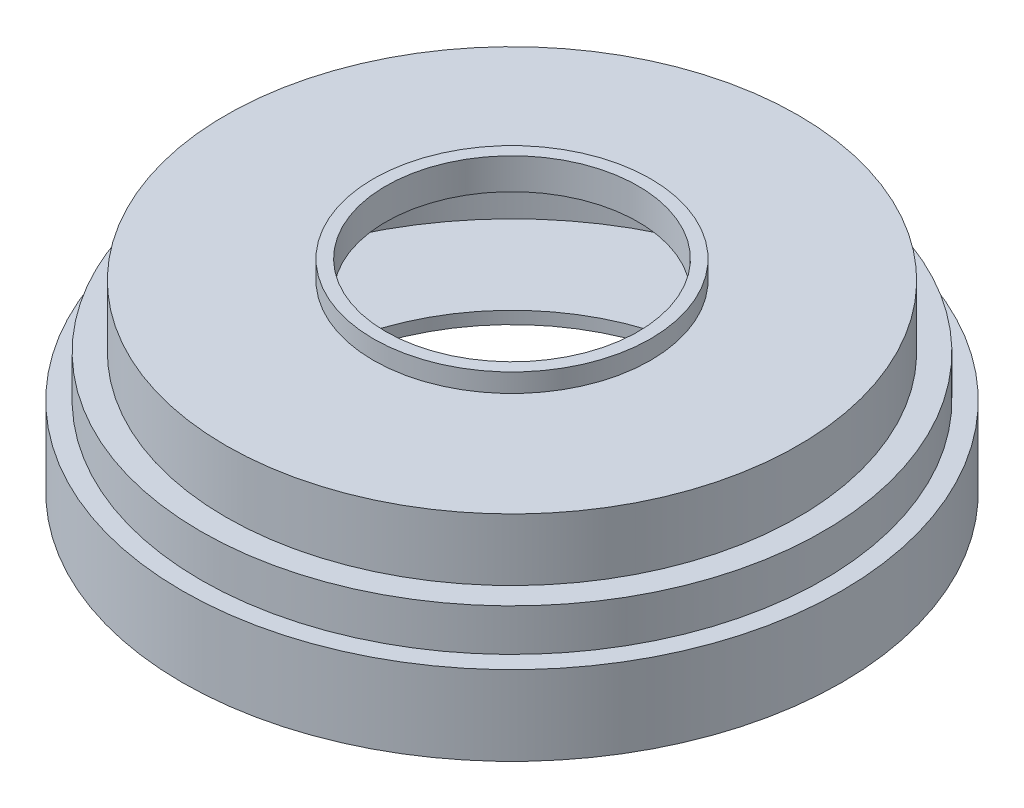
SolidWorks part; units mm, degrees
ref_plane "Front Plane" through (0, 0, 0) normal (0, 0, 1) x (1, 0, 0)
ref_plane "Top Plane" through (0, 0, 0) normal (0, 1, 0) x (1, 0, 0)
ref_plane "Right Plane" through (0, 0, 0) normal (1, 0, 0) x (0, 0, -1)
sketch "Sketch1" plane through (0, 0, 0) normal (0, 0, 1) x (1, 0, 0)
  line L0 (0, 0) -> (0, -21.981) construction
  line L1 (43, 136) -> (43, 141)
  line L2 (-43, 136) -> (43, 136) construction
  line L3 (-55, 136) -> (55, 136) construction
  line L4 (43, 141) -> (-43, 141) construction
  line L5 (60, 141) -> (-60, 141) construction
  line L6 (43, 141) -> (53, 141)
  line L7 (53, 141) -> (53, 153.7728)
  line L9 (53, 153.7728) -> (50, 153.7728)
  line L10 (50, 153.7728) -> (50, 160.5319)
  line L11 (63.1935, 160.5319) -> (-63.1935, 160.5319) construction
  line L12 (50, 160.5319) -> (46, 160.5319)
  line L13 (46, 160.5319) -> (46, 170.5)
  line L14 (106, 170.5) -> (-106, 170.5) construction
  line L15 (46, 170.5) -> (22.2841, 170.5)
  line L16 (22.2841, 170.5) -> (22.2841, 173.5)
  line L17 (41, 136) -> (41, 141)
  line L18 (41, 143) -> (51, 143)
  line L19 (51, 143) -> (51, 151.7728)
  line L20 (51, 151.7728) -> (48, 151.7728)
  line L21 (48, 151.7728) -> (48, 158.5319)
  line L22 (48, 158.5319) -> (44, 158.5319)
  line L23 (44, 158.5319) -> (44, 168.5)
  line L24 (44, 168.5) -> (20.2841, 168.5)
  line L25 (20.2841, 168.5) -> (20.2841, 173.5)
  line L26 (22.2841, 173.5) -> (20.2841, 173.5)
  line L27 (43, 136) -> (41, 136)
  line L29 (41, 143) -> (33, 143)
  line L31 (41, 141) -> (33, 141)
  line L32 (33, 143) -> (33, 141)
  line L33 (41, 136) -> (41, 143) construction
  dimension "D1" = 2
revolve "Revolve1" add sketch "Sketch1" angle 360 about L0
